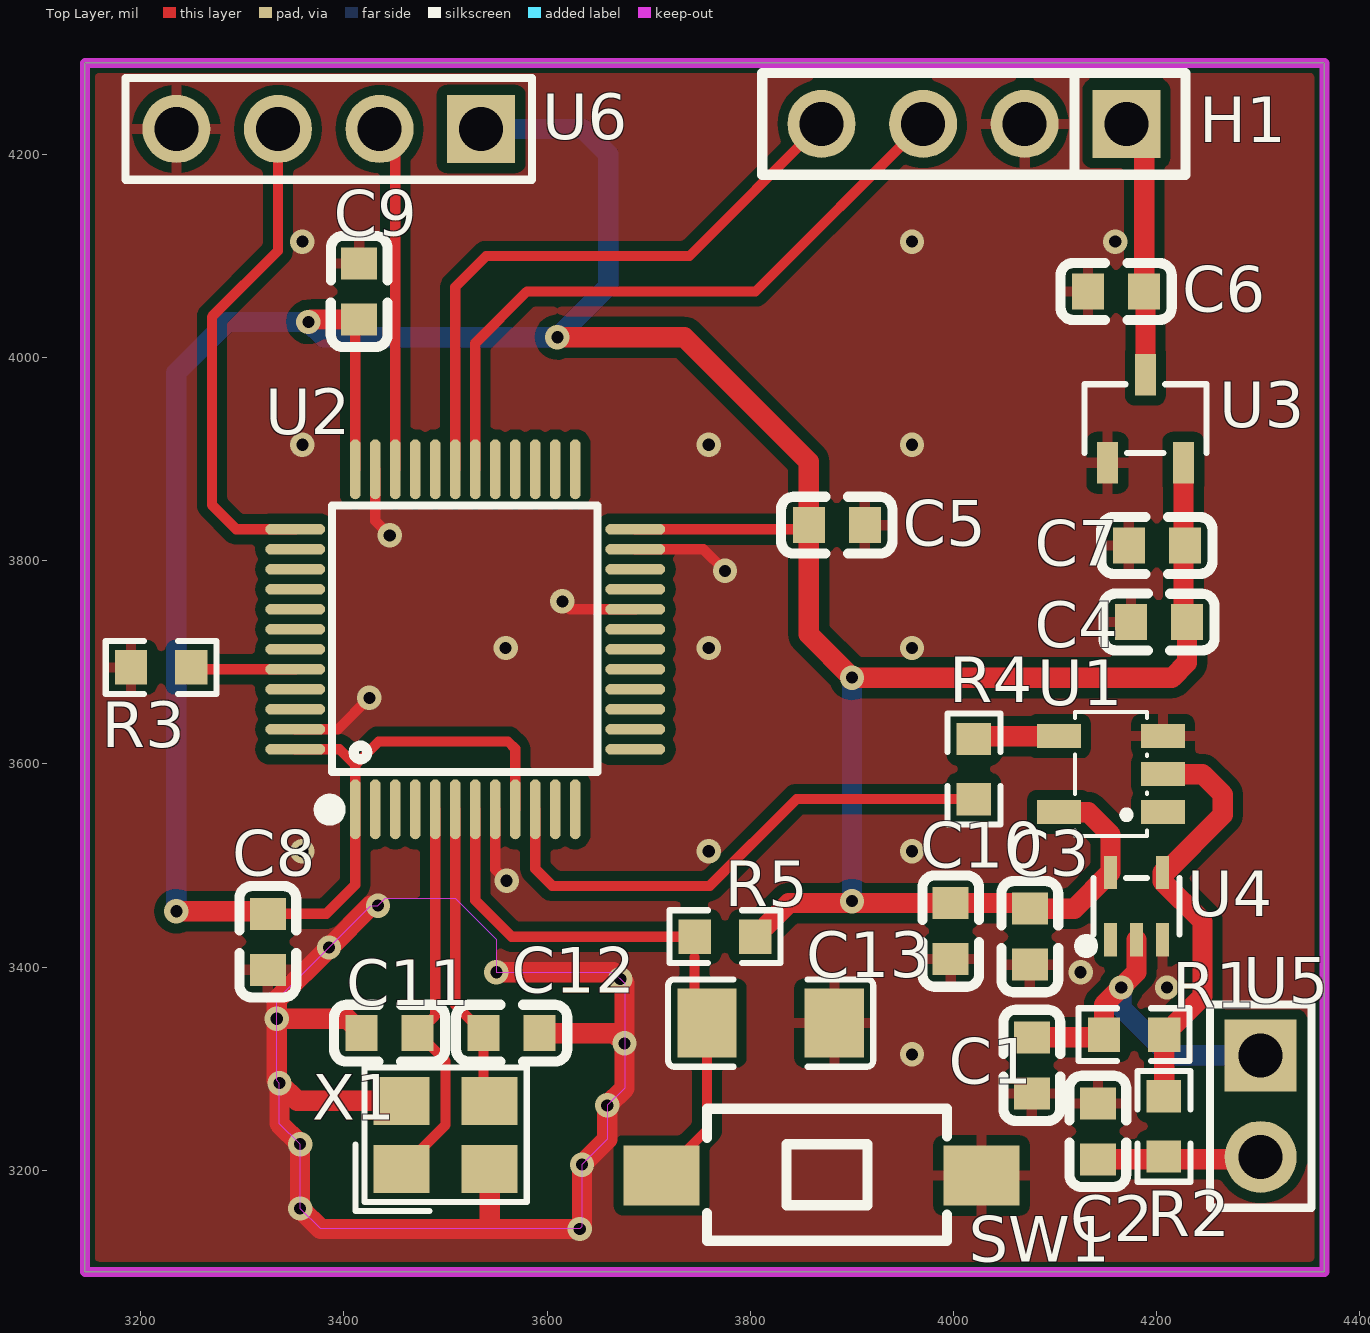
[diagram p0: Top Layer view]
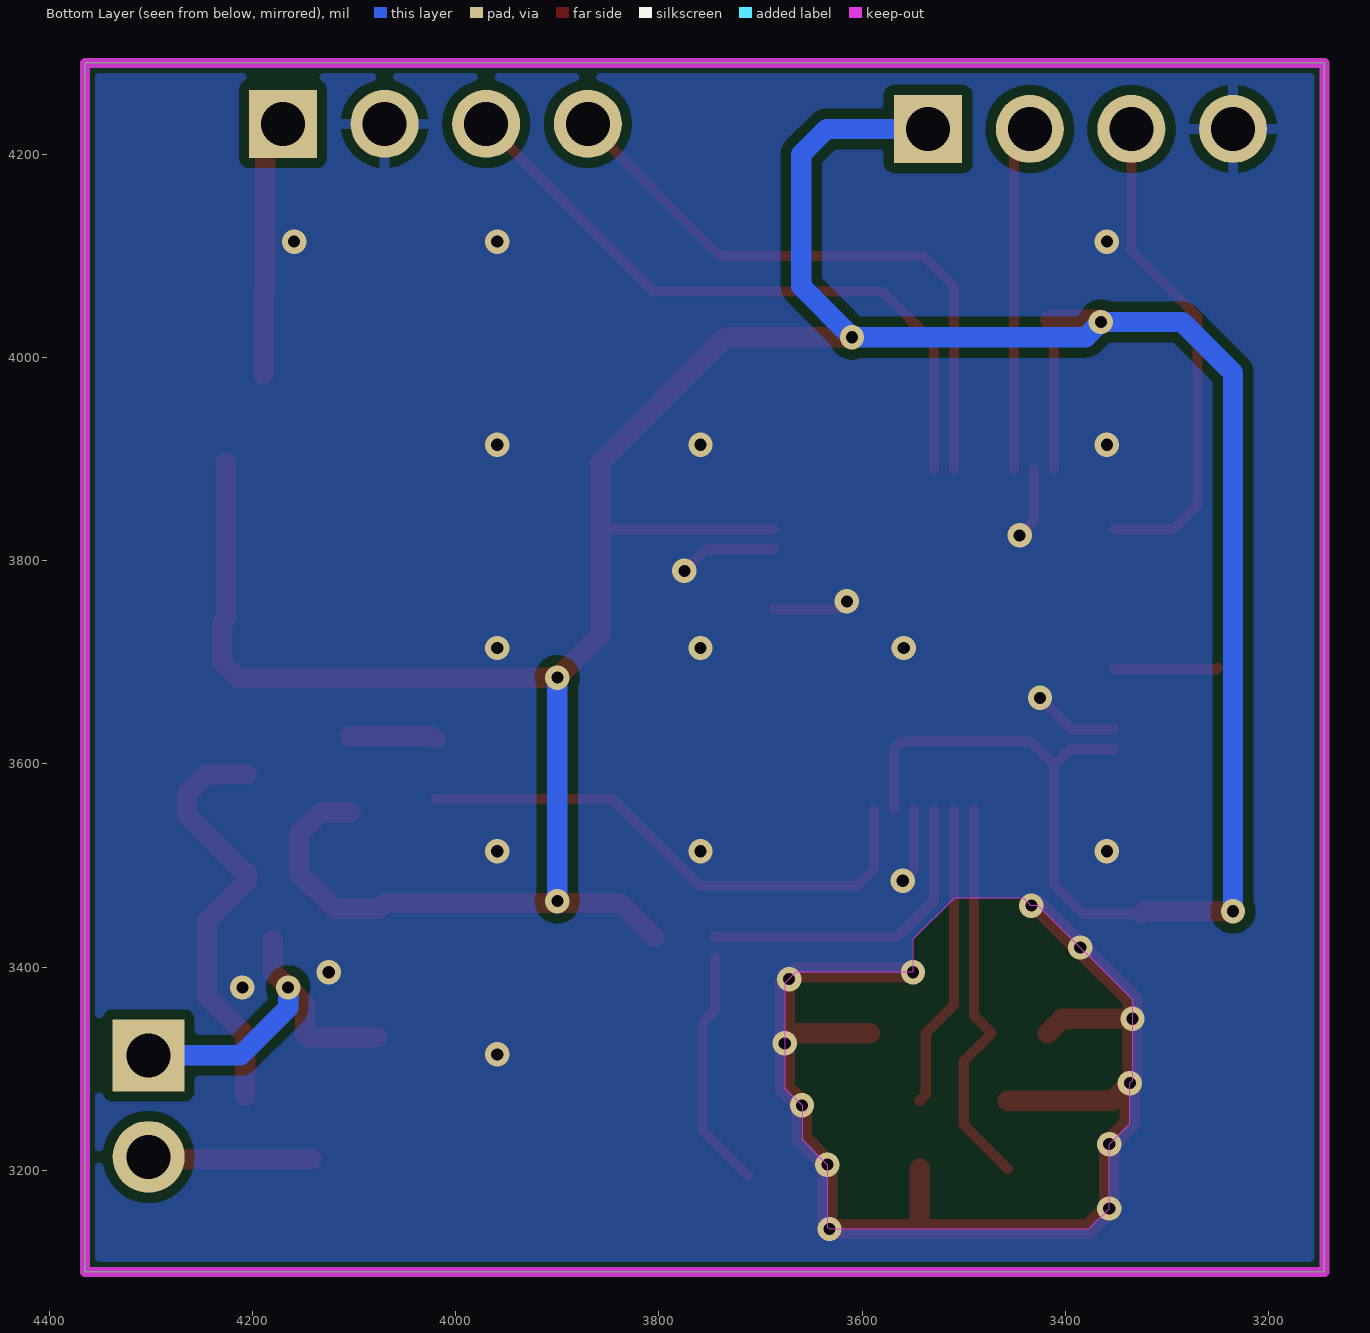
[diagram p1: Bottom Layer view, seen from below]
# Altium PCB MISC51896.pcbdoc
Units mil, origin at the board's own origin, x right, y up, seen from the top; angles counter-clockwise.
Board outline 1220 x 1190 mil, 2 copper layers (Top Layer, Bottom Layer), stack 62.206 mil thick; 27 components, 16 nets, 113 pads, 38 vias.

## Layer stack, top to bottom
Top Solder Mask Layer: solder mask 0.394, Dk 3.3
Top Layer: signal copper 1.379
Dielectric1: surface 59.449, FR4, Dk 4.5
Bottom Layer: signal copper 1.378
Bottom Solder Mask Layer: solder mask 0.394, Dk 3.3

## Board outline
3145,4290 3145,3100 4365,3100 4365,4290

## Design rules (kind name [scope] priority, off if disabled: settings)
BoardOutlineClearance copperThickness2oz_1 [All] p2 off: genericclearance=7.99 ignorepadtopadclearanceinfootprint=FALSE except(0: Arc-SplitContinuation Track-SplitContinuation SMDPad-SplitContinuation THPad-SplitContinuation Via-SplitContinuation Fill-SplitContinuation Region-SplitContinuation Poly-SplitContinuation Text-SplitContinuation Hole-SplitContinuation; 5.98: Arc-CutoutEdge SMDPad-CutoutEdge THPad-CutoutEdge Via-CutoutEdge Fill-CutoutEdge Region-CutoutEdge Text-CutoutEdge; 6.93: Hole-OutlineEdge Hole-CutoutEdge; 10: Poly-OutlineEdge Poly-CutoutEdge; 11.81: Arc-OutlineEdge Track-OutlineEdge SMDPad-OutlineEdge THPad-OutlineEdge Via-OutlineEdge Fill-OutlineEdge Region-OutlineEdge Text-OutlineEdge Track-CutoutEdge)
BoardOutlineClearance copperThickness1oz_1 [All] p4: genericclearance=4.02 ignorepadtopadclearanceinfootprint=FALSE except(0: Arc-SplitContinuation Track-SplitContinuation SMDPad-SplitContinuation THPad-SplitContinuation Via-SplitContinuation Fill-SplitContinuation Region-SplitContinuation Poly-SplitContinuation Text-SplitContinuation Hole-SplitContinuation; 6: SMDPad-CutoutEdge THPad-CutoutEdge Via-CutoutEdge Fill-CutoutEdge Region-CutoutEdge Text-CutoutEdge; 6.93: Hole-OutlineEdge Hole-CutoutEdge; 10: Poly-OutlineEdge Poly-CutoutEdge; 11.8: Arc-OutlineEdge Track-OutlineEdge SMDPad-OutlineEdge THPad-OutlineEdge Via-OutlineEdge Fill-OutlineEdge Region-OutlineEdge Text-OutlineEdge; 11.81: Arc-CutoutEdge Track-CutoutEdge)
Clearance copperThickness2oz [All] p1 off: gap=7.99 ignorepadtopadclearanceinfootprint=FALSE except(5.98: SMDPad-Track SMDPad-SMDPad THPad-Track SMDPad-THPad THPad-THPad Track-Via SMDPad-Via THPad-Via Via-Via Fill-Track Region-Track Fill-SMDPad Region-SMDPad Fill-THPad Region-THPad Fill-Via Region-Via Fill-Fill Fill-Region Region-Region Arc-Track Arc-SMDPad Arc-THPad Arc-Via Fill-Arc Region-Arc Arc-Arc Text-Track SMDPad-Text Text-THPad Text-Via Fill-Text Region-Text Arc-Text Text-Text; 6.93: Hole-Track Hole-SMDPad Hole-THPad Hole-Via Fill-Hole Region-Hole Hole-Arc Hole-Text; 10: Poly-Track Poly-SMDPad Poly-THPad Poly-Via Poly-Fill Poly-Region Poly-Poly Poly-Arc Poly-Text Poly-Hole)
Clearance copperThickness1oz [All] p3: gap=4.02 ignorepadtopadclearanceinfootprint=FALSE except(5.98: SMDPad-Track SMDPad-SMDPad THPad-Track SMDPad-THPad THPad-THPad Track-Via SMDPad-Via THPad-Via Via-Via Fill-Track Region-Track Fill-SMDPad Region-SMDPad Fill-THPad Region-THPad Fill-Via Region-Via Fill-Fill Fill-Region Region-Region; 6: Arc-Track Arc-SMDPad Arc-THPad Arc-Via Fill-Arc Region-Arc Arc-Arc Text-Track SMDPad-Text Text-THPad Text-Via Fill-Text Region-Text Arc-Text Text-Text; 6.93: Hole-Track Hole-SMDPad Hole-THPad Hole-Via Fill-Hole Region-Hole Hole-Arc Hole-Text; 10: Poly-Track Poly-SMDPad Poly-THPad Poly-Via Poly-Fill Poly-Region Poly-Poly Poly-Arc Poly-Text Poly-Hole)
DiffPairsRouting differentialPair [All] p1: maxlimit=6 minlimit=6 mostfreqgap=6 toplayer_minwidth=5 toplayer_prefwidth=10 toplayer_maxwidth=100 toplayer_mingap=6 toplayer_prefgap=6 toplayer_maxgap=6 bottomlayer_minwidth=5 bottomlayer_prefwidth=10 bottomlayer_maxwidth=100 bottomlayer_mingap=6 bottomlayer_prefgap=6 bottomlayer_maxgap=6 maxuncoupledlength=10
HoleToHoleClearance otherClearance [All] p1: gap=11.81 allowstackedmicrovias=TRUE
Length netLength [All] p1: minlimit=0 maxlimit=0
MatchedLengths netLengthTolerance [All] p1: tolerance=1000
PasteMaskExpansion pasteMaskExpansion [All] p1: expansion=0
PlaneConnect innerPlane [All] p1: planeconnectstyle=Relief reliefexpansion=20 reliefentries=4 reliefconductorwidth=10 reliefairgap=10
PolygonConnect copperRegion [(InNet('GND'))] p1: connectstyle=Relief reliefconductorwidth=10 reliefentries=4 polygonreliefangle="90 Angle" airgapwidth=10 via.connectstyle=Relief via.reliefconductorwidth=10 via.reliefentries=4 via.polygonreliefangle="90 Angle" via.airgapwidth=10
RoutingVias viaSize [All] p1: holewidth=12.01 width=24.02 viastyle="Through Hole" minholewidth=11.81 minwidth=19.68 maxholewidth=248.03 maxwidth=393.7
SolderMaskExpansion solderMaskExpansion [IsVia] p1: expansion=-1000 istentingtop=TRUE
SolderMaskExpansion solderMaskExpansion [All] p2: expansion=2 istentingtop=FALSE
Width copperThickness2oz_2 [All] p1 off: maxlimit=100 minlimit=8 preferedwidth=10
Width copperThickness1oz_2 [All] p2: maxlimit=100 minlimit=5 preferedwidth=10

## Components (designator, comment, footprint, x,y, rotation, side; value= is the part's Value field where it differs from the comment)
C1 "33pF" C0603 4077,3303.35 r270 top
C2 "33pF" C0603 4142,3238.35 r90 top
C3 "100nF" C0603 4075,3430 r90 top
C4 "100nF" C0603 4202.12,3739.65 r180 top
C5 "100nF" C0603 3885,3835 r180 top
C6 "1uF" C0603 4160,4065 r0 top
C7 "10uF" C0603 4200,3815 r0 top
C8 "100nF" C0603 3325,3425 r90 top
C9 "100nF" C0603 3415,4065 r90 top
C10 "100nF" C0603 3997.2,3435.5 r90 top
C11 "20pF" C0603 3445,3335 r180 top
C12 "20pF" C0603 3565,3335 r0 top
C13 "100uF" C1206 3820,3345 r180 top
H1 "2.54-1*4P female" HDR-TH_4P-P2.54-V-F 4020,4230 r180 top
R1 "1MΩ" R0603 4177.65,3333.52 r0 top
R2 "510Ω" R0603 4207,3243.35 r270 top
R3 "10kΩ" R0603 3220,3695 r180 top
R4 "33Ω" R0603 4020,3595 r90 top
R5 "1kΩ" R0603 3775,3430 r0 top
SW1 "TS-1101-C-W" SW-SMD_L6.0-W3.3-LS8.0 3870,3195 r180 top
U1 "SN74LVC1G14DBVR" SOT-23-5_L3.0-W1.7-P0.95-LS2.8-BR 4155,3590 r0 top
U2 "STM32F103C8T6" LQFP-48_L7.0-W7.0-P0.50-LS9.0-BL 3519.34,3722.72 r0 top
U3 "XC6206P332MR" SOT-23-3_L3.0-W1.7-P0.95-LS2.9-BR 4188.83,3939.89 r270 top
U4 "SN74LVC1GU04DCKR" SC-70-5_L2.1-W1.3-P0.65-LS2.1-BL 4180,3460 r0 top
U5 "HX PZ2.54-1x2P ZZ" HDR-TH_2P-P2.54-V-M-3 4302.31,3263.18 r270 top
U6 "2541WV-04P" HDR-TH_4P-P2.54-V-M-1 3385,4225 r180 top
X1 "8MHz" CRYSTAL-SMD_4P-L3.2-W2.5-BL 3500,3235 r0 top

## Footprints (in the part's own frame and the unit in brackets; to place one, negate y for a bottom-side part, rotate by r counter-clockwise, add the part's x,y. Pads: shape width x height; smd on the part's side, far side on the other; paste and mask are expansions set on the pad)
C0603 [mm]
  rect 0.8x0.9 smd: 1(-0.7,0) 2(0.7,0)
  silkscreen extent -1.39,-0.71 1.39,0.71
C1206 [mm]
  rect 1.485x1.728 smd paste-100 mask+0.051: 1(-1.593,0) 2(1.593,0)
  silkscreen extent -2.56,-1.09 2.56,1.09
CRYSTAL-SMD_4P-L3.2-W2.5-BL [mm]
  rect 1.4x1.2 smd: 1(-1.1,-0.85) 2(1.1,-0.85) 3(1.1,0.85) 4(-1.1,0.85)
  silkscreen extent -2.26,-1.91 2.03,1.68
HDR-TH_2P-P2.54-V-M-3 [mm]
  rect 1.8x1.8 hole 1.1: 1(-1.27,0)
  round 1.8 hole 1.1: 2(1.27,0)
  silkscreen extent -2.54,-1.27 2.54,1.27
HDR-TH_4P-P2.54-V-F [mm]
  rect 1.7x1.7 hole 1.1: 1(-3.81,0)
  round 1.7 hole 1.1: 2(-1.27,0) 3(1.27,0) 4(3.81,0)
  silkscreen extent -5.29,-1.27 5.29,1.27
HDR-TH_4P-P2.54-V-M-1 [mm]
  rect 1.7x1.7 hole 1.1: 1(-3.81,0)
  round 1.7 hole 1.1: 2(-1.27,0) 3(1.27,0) 4(3.81,0)
  silkscreen extent -5.08,-1.27 5.08,1.27
LQFP-48_L7.0-W7.0-P0.50-LS9.0-BL [mm]
  oval 0.27x1.5 smd paste+0 mask+0.05: 1(-2.75,-4.25) 2(-2.25,-4.25) 3(-1.75,-4.25) 4(-1.25,-4.25) 5(-0.75,-4.25) 6(-0.25,-4.25) 7(0.25,-4.25) 8(0.75,-4.25) 9(1.25,-4.25) 10(1.75,-4.25) 11(2.25,-4.25) 12(2.75,-4.25) 25(2.75,4.25) 26(2.25,4.25) 27(1.75,4.25) 28(1.25,4.25) 29(0.75,4.25) 30(0.25,4.25) 31(-0.25,4.25) 32(-0.75,4.25) 33(-1.25,4.25) 34(-1.75,4.25) 35(-2.25,4.25) 36(-2.75,4.25)
  oval 1.5x0.27 smd paste+0 mask+0.05: 13(4.25,-2.75) 14(4.25,-2.25) 15(4.25,-1.75) 16(4.25,-1.25) 17(4.25,-0.75) 18(4.25,-0.25) 19(4.25,0.25) 20(4.25,0.75) 21(4.25,1.25) 22(4.25,1.75) 23(4.25,2.25) 24(4.25,2.75) 37(-4.25,2.75) 38(-4.25,2.25) 39(-4.25,1.75) 40(-4.25,1.25) 41(-4.25,0.75) 42(-4.25,0.25) 43(-4.25,-0.25) 44(-4.25,-0.75) 45(-4.25,-1.25) 46(-4.25,-1.75) 47(-4.25,-2.25) 48(-4.25,-2.75)
  silkscreen extent -3.59,-4.46 3.3,3.34
R0603 [mil]
  rect 31.75x34.02 smd paste-3937.01 mask+2: 1(-29.66,0) 2(29.66,0)
  silkscreen extent -55,-26 55,26
SC-70-5_L2.1-W1.3-P0.65-LS2.1-BL [mm]
  rect 0.315x0.835 smd: 1(-0.65,-0.843) 2(0,-0.843) 3(0.65,-0.843) 4(0.65,0.842) 5(-0.65,0.842)
  silkscreen extent -1.41,-1.14 1.08,0.7
SOT-23-3_L3.0-W1.7-P0.95-LS2.9-BR [mil]
  rect 40.85x20.95 smd: 1(43.36,-37.4) 2(43.36,37.4) 3(-43.36,0)
  silkscreen extent -34,-60 34,60
SOT-23-5_L3.0-W1.7-P0.95-LS2.8-BR [mm]
  rect 1.1x0.6 smd: 1(1.3,-0.95) 2(1.3,0) 3(1.3,0.95) 4(-1.3,0.95) 5(-1.3,-0.95)
  silkscreen extent -0.9,-1.55 0.9,1.55
SW-SMD_L6.0-W3.3-LS8.0 [mm]
  rect 1.9x1.5 smd: 1(-4,0) 2(4,0)
  silkscreen extent -3.14,-1.67 2.86,1.63

## Via types
v1: diameter 24.02, hole 12, Top Layer to Bottom Layer, 38 vias

## Nets (pads, with @x,y where several pads share a name; then routed paths per layer and width w, separated by ;. In a path a pad name is that pad's centre, name@x,y a point inside that pad or via, vN(x,y) a via of type N, cw(c..) or ccw(c..) an arc to the next point about the centre after c; other vN are vias at no path point)
3.3V: C3.2 C4.1 C5.2 C7.2 C8.2 C9.1 C10.2 R5.2 U1.5 U2.1 U2.9 U2.24 U2.36 U2.48 U3.2 U4.5 U6.1 | length 4005
  Top Layer w10: C8.2 3382.56,3452.56 3411.07,3481.07 U2.1 3411.07,3598.93 ; U2.48 3395.55,3614.45 3411.07,3598.93 ; U2.36 3411.07,4033.51 C9.1 ; U2.9 3568.55,3615 3561.48,3622.07 3434.22,3622.07 3411.07,3598.93 ; U2.24 3853.43,3830.99 C5.2
  Top Layer w20: v1(3235,3455) 3322.56,3455 C8.2 ; v1(3365,4035) 3367.44,4037.44 C9.1 ; v1(3610,4020) 3735,4020 3857.44,3897.56 C5.2 3857.44,3727.56 v1(3900,3685) 4215,3685 4229.68,3699.68 C4.1 4226.23,3743.1 U3.2 ; R5.2 3837.72,3463.06 v1@3901.94,3463.06 ; v1(3900,3465) v1@3901.94,3463.06 ; U1.5 4132.4,3552.6 4154.4,3530.6 U4.5 4118.8,3457.56 C3.2 4069.5,3463.06 C10.2 v1@3901.94,3463.06
  Bottom Layer w20: v1(3235,3455) 3235,3985 3285,4035 v1(3365,4035) 3380,4020 v1(3610,4020) 3660,4070 3660,4200 3635,4225 U6.1 ; v1(3900,3465) v1(3900,3685)
5V-IN: C6.2 H1.1 U3.3 | length 254.6
  Top Layer w20: H1.1 4187.56,4212.44 C6.2 4188.83,4063.73 U3.3
34: U2.34 U6.2 | length 341.4
  Top Layer w10: U6.2 3450.44,4209.56 U2.34
37: U2.37 U6.3 | length 488.9
  Top Layer w10: U6.3 3335,4105 3270,4040 3270,3855 3294.01,3830.99 U2.37
$1N12: R1.2 R2.1 U1.2 U4.4 | length 422.3
  Top Layer w20: U1.2 4245,3590 4265,3570 4265,3550 4208.17,3493.17 U4.4 4205.59,3484.41 4245,3445 4245,3371.21 R1.2 4207.31,3273.32 R2.1
$1N15: C2.1 R2.2 U5.2 | length 161.3
  Top Layer w20: C2.1 4299.92,3210.79 U5.2
$1N30: C1.1 R1.1 U4.2 U5.1 | length 355.3
  Top Layer w20: C1.1 4145.38,3330.91 R1.1 4147.99,3362.99 v1(4165,3380) 4180,3395 U4.2
  Bottom Layer w20: v1(4165,3380) 4165,3360 4211.82,3313.18 U5.1
$1N53: R3.1 U2.44 | length 103.1
  Top Layer w10: R3.1 3251.47,3693.19 U2.44
$1N64: R4.2 U1.4 | length 84.9
  Top Layer w20: R4.2 4022.74,3627.4 U1.4
GND: C1.2 C2.2 C3.1 C4.2 C5.1 C6.1 C7.1 C8.1 C9.2 C10.1 C11.2 C12.2 C13.1 H1.2 R3.2 SW1.1 U1.3 U2.8 U2.20 U2.23 U2.35 U2.47 U3.1 U4.3 U6.4 X1.2 X1.4 | length 1794.7
  Top Layer w10: U2.47 3394.14,3634.14 v1(3425,3665) ; U2.35 3430.76,3839.24 v1(3445,3825) ; U2.8 3548.87,3496.13 v1(3560,3485) ; v1(3615,3760) 3622.75,3752.25 U2.20 ; U2.23 3753.7,3811.3 v1(3775,3790)
  Top Layer w20: C11.2 3403.24,3349.2 v1(3333.9,3349.2) ; v1(3433.44,3460.54) 3426.49,3460.54 v1(3385.28,3419.33) 3333.9,3367.95 v1(3333.9,3349.2) ; X1.4 3353.91,3268.47 v1(3336.51,3285.87) ; 3543.31,3142.33 X1.2 ; v1(3550,3395) 3665.18,3395 v1(3671.92,3388.25) 3676.1,3384.07 v1(3676.1,3325.01) ; C12.2 3666.11,3335 v1(3676.1,3325.01) ; v1(3333.9,3349.2) 3333.9,3288.48 v1(3336.51,3285.87) ; v1(3336.51,3285.87) 3336.51,3246.05 v1(3356.76,3225.81) v1(3356.76,3162.42) 3376.88,3142.29 3543.28,3142.29 v1(3632.12,3142.29) 3634.24,3144.42 v1(3634.24,3205.64) 3659.17,3230.57 v1(3659.17,3263.92) 3676.1,3280.86 v1(3676.1,3325.01)
  other v1: 3959.1,3314.1 4210,3380 4125,3395 3359.1,3514.1 3759.1,3514.1 3959.1,3514.1 3559.1,3714.1 3759.1,3714.1 3959.1,3714.1 3359.1,3914.1 3759.1,3914.1 3959.1,3914.1 3359.1,4114.1 3959.1,4114.1 4159.1,4114.1
OSC_IN: C11.1 U2.5 X1.1 | length 390.3
  Top Layer w10: X1.1 3500,3244.84 3500,3307.56 C11.1 3489.81,3352.25 U2.5
OSC_OUT: C12.1 U2.6 X1.3 | length 300.9
  Top Layer w10: U2.6 3509.5,3362.94 C12.1 3537.44,3274.34 X1.3
QCM_10MHZ_OUT: R4.1 U2.10 | length 532.7
  Top Layer w10: U2.10 3588.24,3496.76 3605,3480 3760,3480 3845.34,3565.34 R4.1
REST: C13.2 R5.1 SW1.2 U2.7 | length 559.2
  Top Layer w10: U2.7 3529.18,3465.82 3565,3430 R5.1 ; SW1.2 3757.3,3239.78 C13.2 3745,3357.3 3745,3410
RX: H1.4 U2.31 | length 606.4
  Top Layer w10: U2.31 3509.5,4069.5 3540,4100 3740,4100 H1.4
TX: H1.3 U2.30 | length 654.3
  Top Layer w10: U2.30 3529.18,4014.18 3580,4065 3805,4065 H1.3
pads on no net: U1.1 U2.2 U2.3 U2.4 U2.11 U2.12 U2.13 U2.14 U2.15 U2.16 U2.17 U2.18 U2.19 U2.21 U2.22 U2.25 U2.26 U2.27 U2.28 U2.29 U2.32 U2.33 U2.38 U2.39 U2.40 U2.41 U2.42 U2.43 U2.45 U2.46 U4.1

## Polygon pours and split planes (outlines as drawn)
GND on Top Layer (solid, remove dead copper, pour order 0): 3020,4390 3020,3000 4475,3000 4475,4390
GND on Bottom Layer (solid, remove dead copper, pour order 2): 3000,4350 3000,3080 4555,3080 4555,4350

## Keep-outs
Board Outline Layer:
  region: 3433.44,3460.54 3440.84,3467.94 3509.5,3467.94 3550,3427.45 3550,3395 3665.18,3395 3676.1,3384.07 3676.1,3280.86 3659.17,3263.92 3659.17,3230.57 3634.24,3205.64 3634.24,3144.42 3632.12,3142.29 3376.88,3142.29 3356.76,3162.42 3356.76,3225.81 3336.51,3246.05 3336.51,3285.87 3333.9,3288.48 3333.9,3367.95 3426.49,3460.54
  lines w10: 3145,3100 3145,4290 4365,4290 4365,3100 3145,3100